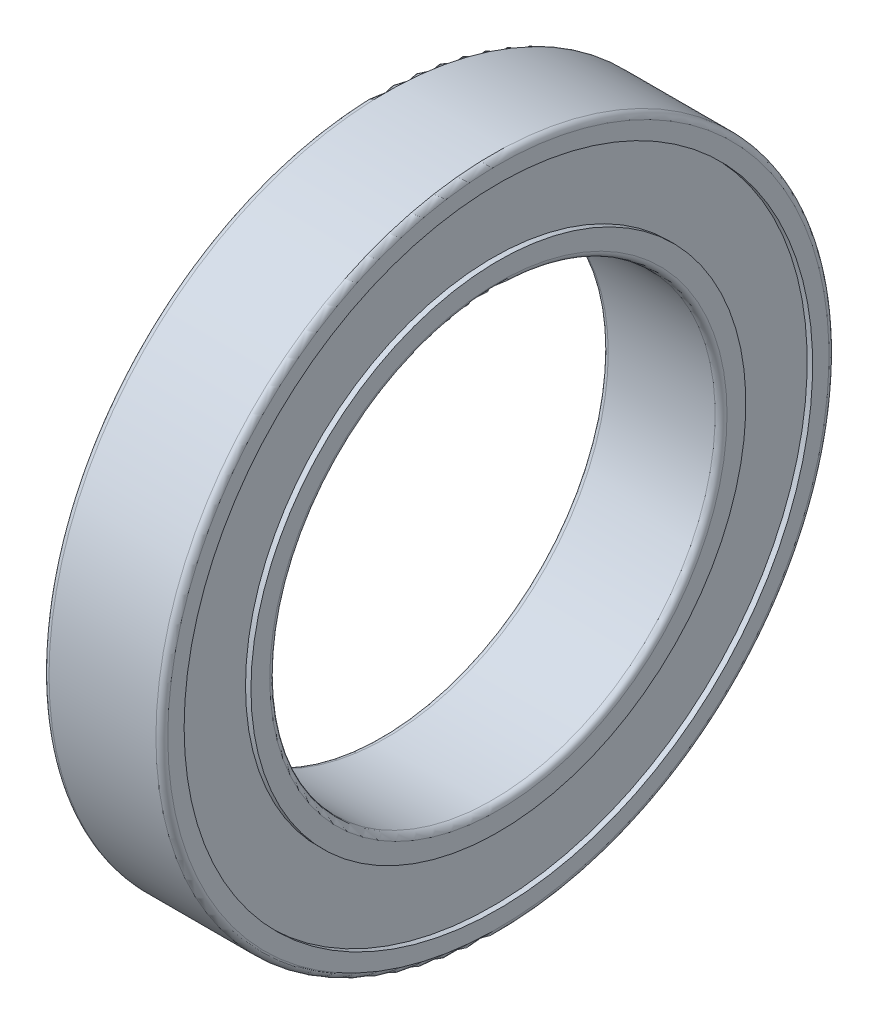
SolidWorks part; units mm, degrees
ref_plane "Front Plane" through (0, 0, 0) normal (0, 0, 1) x (1, 0, 0)
ref_plane "Top Plane" through (0, 0, 0) normal (0, 1, 0) x (1, 0, 0)
ref_plane "Right Plane" through (0, 0, 0) normal (1, 0, 0) x (0, 0, -1)
sketch "Sketch1" plane through (0, 0, 0) normal (0, 0, 1) x (1, 0, 0)
  line L0 (0, 0) -> (12, 0) construction
  line L1 (0, 22.5) -> (12, 22.5)
  line L2 (0, 34) -> (12, 34)
  line L3 (0, 34) -> (0, 31.75)
  line L4 (0, 31.75) -> (0.55, 31.75)
  line L5 (12, 34) -> (12, 31.75)
  line L6 (0.55, 31.75) -> (0.55, 25)
  line L7 (0.55, 25) -> (0, 25)
  line L8 (0, 25) -> (0, 22.5)
  line L9 (12, 31.75) -> (11.45, 31.75)
  line L10 (11.45, 31.75) -> (11.45, 25)
  line L11 (11.45, 25) -> (12, 25)
  line L12 (12, 25) -> (12, 22.5)
  dimension "D" = 68
  dimension "B" = 12
  dimension "D_s" = 45
  dimension "MSM_1" = 63.5
  dimension "MSM_2" = 50
  dimension "MSM_3" = 0.55
revolve "Revolve1" add sketch "Sketch1" angle 360 about L0
fillet "Fillet1" radius 0.6 2 edges at (12, 0, 34) (0, 0, 34)
fillet "Fillet2" radius 0.6 2 edges at (12, 0, 22.5) (0, 0, 22.5)
